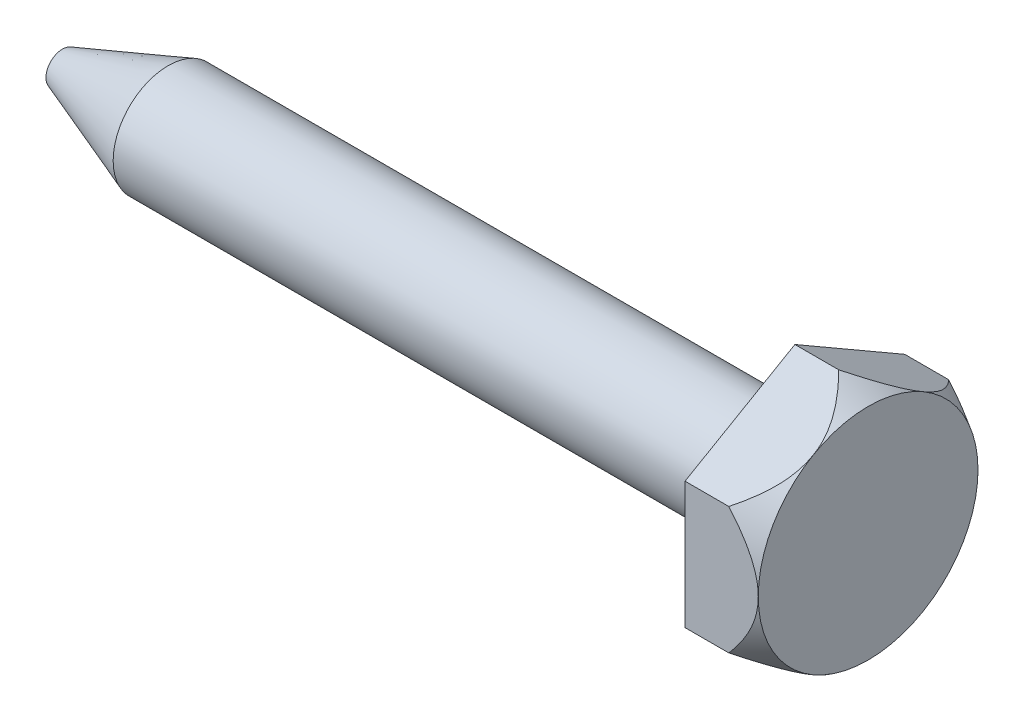
from build123d import *

# Parameters (mm, degrees)
BOSS_EXTRUDE1_DEPTH = 4
SKETCH2_OUTSIDE_W   = 22.372
SKETCH2_OUTSIDE_H   = 24.228
SKETCH2_OUTSIDE_R   = 6
CUT_EXTRUDE1_DEPTH  = 4
CUT_EXTRUDE1_DRAFT  = -30


with BuildPart() as part:
    # Sketch1 → Boss-Extrude1 (new body)
    with BuildSketch(Plane(origin=(0, 0, 0), x_dir=(0, 0, -1), z_dir=(1, 0, 0))):
        Polygon((0, -6.92820323), (6, -3.464101615), (6, 3.464101615), (0, 6.92820323), (-6, 3.464101615), (-6, -3.464101615), align=None)
    extrude(amount=BOSS_EXTRUDE1_DEPTH)


with BuildPart() as cut_extrude1_tool:
    # Sketch2 outside → Cut-Extrude1 (with draft: the straight prism first)
    with BuildSketch(Plane(origin=(4, 0, 0), x_dir=(0, 0, -1), z_dir=(1, 0, 0))):
        Rectangle(SKETCH2_OUTSIDE_W, SKETCH2_OUTSIDE_H)
        Circle(SKETCH2_OUTSIDE_R, mode=Mode.SUBTRACT)
    extrude(amount=-CUT_EXTRUDE1_DEPTH)
    # Cut-Extrude1: the draft: its side faces are tilted about the plane it starts from
    cut_extrude1_sides = [cut_extrude1_tool.faces().sort_by_distance(p)[0] for p in [
        (2, -12.114, 0),
        (2, 0, -11.186),
        (2, 12.114, 0),
        (2, 0, 11.186),
        (2, 0, 6),
    ]]
    draft(cut_extrude1_sides, Plane(origin=(4, 0, 0), x_dir=(0, 0, -1), z_dir=(1, 0, 0)), CUT_EXTRUDE1_DRAFT)


with BuildPart() as part_1:
    add(part.part)

    # Cut-Extrude1: cut by cut_extrude1_tool
    add(cut_extrude1_tool.part, mode=Mode.SUBTRACT)

    # Sketch3 → Revolve1 (revolve)
    with BuildSketch(Plane.XY, mode=Mode.PRIVATE) as revolve1_sk:
        Polygon((0, 3), (0, 0), (-40, 0), (-40, 0.9), (-34.230297419, 3), align=None)
    revolve(revolve1_sk.sketch.rotate(Axis((-29.866000922, 0, 0), (1, 0, 0)), 90), axis=Axis((-29.866000922, 0, 0), (1, 0, 0)))


solid = part_1.part
